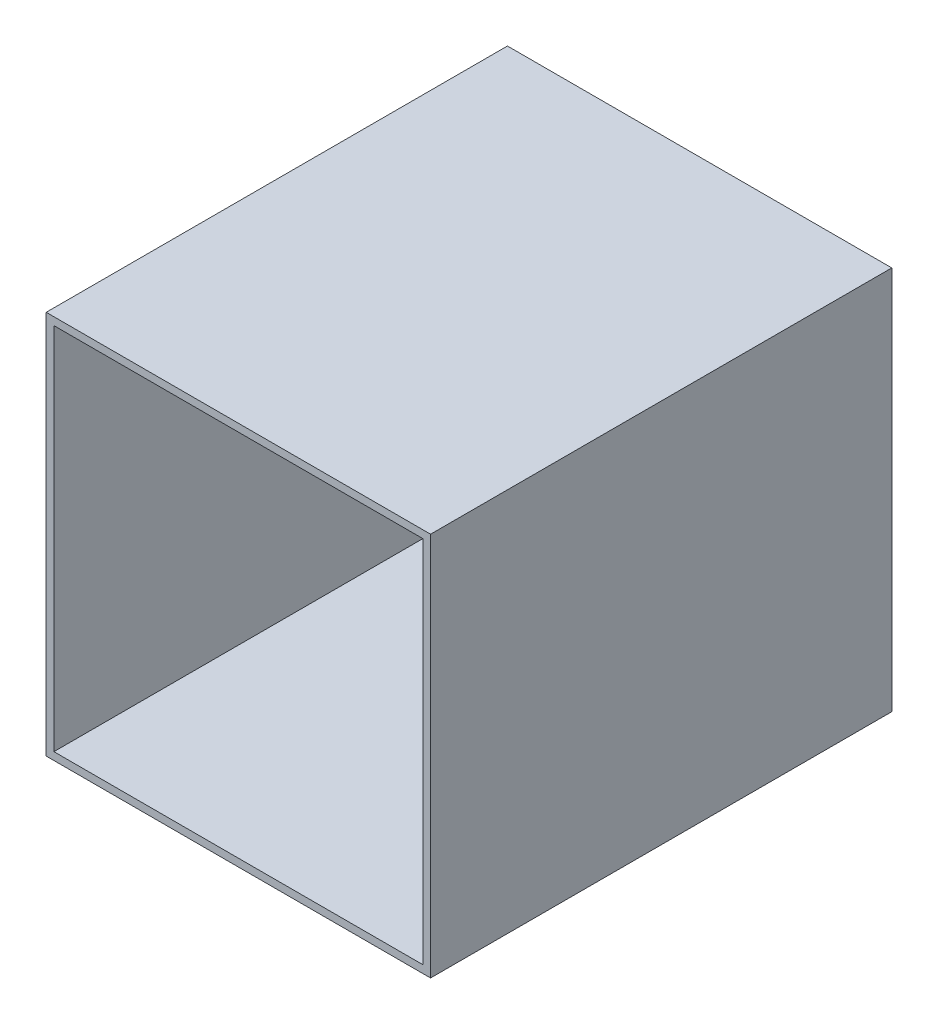
SolidWorks part; units mm, degrees
ref_plane "Front Plane" through (0, 0, 0) normal (0, 0, 1) x (1, 0, 0)
ref_plane "Top Plane" through (0, 0, 0) normal (0, 1, 0) x (1, 0, 0)
ref_plane "Right Plane" through (0, 0, 0) normal (1, 0, 0) x (0, 0, -1)
other "Configuration Table"
sketch "Sketch1" plane through (0, 0, 0) normal (0, 0, 1) x (1, 0, 0)
  line L1 (0, 0) -> (500, 0)
  line L2 (0, 0) -> (0, 500)
  line L3 (0, 500) -> (500, 500)
  line L4 (500, 0) -> (500, 500)
  dimension "D1" = 500
  dimension "D2" = 500
extrude "Boss-Extrude1" add sketch "Sketch1" along normal blind 600
shell "Shell1" thickness 10
